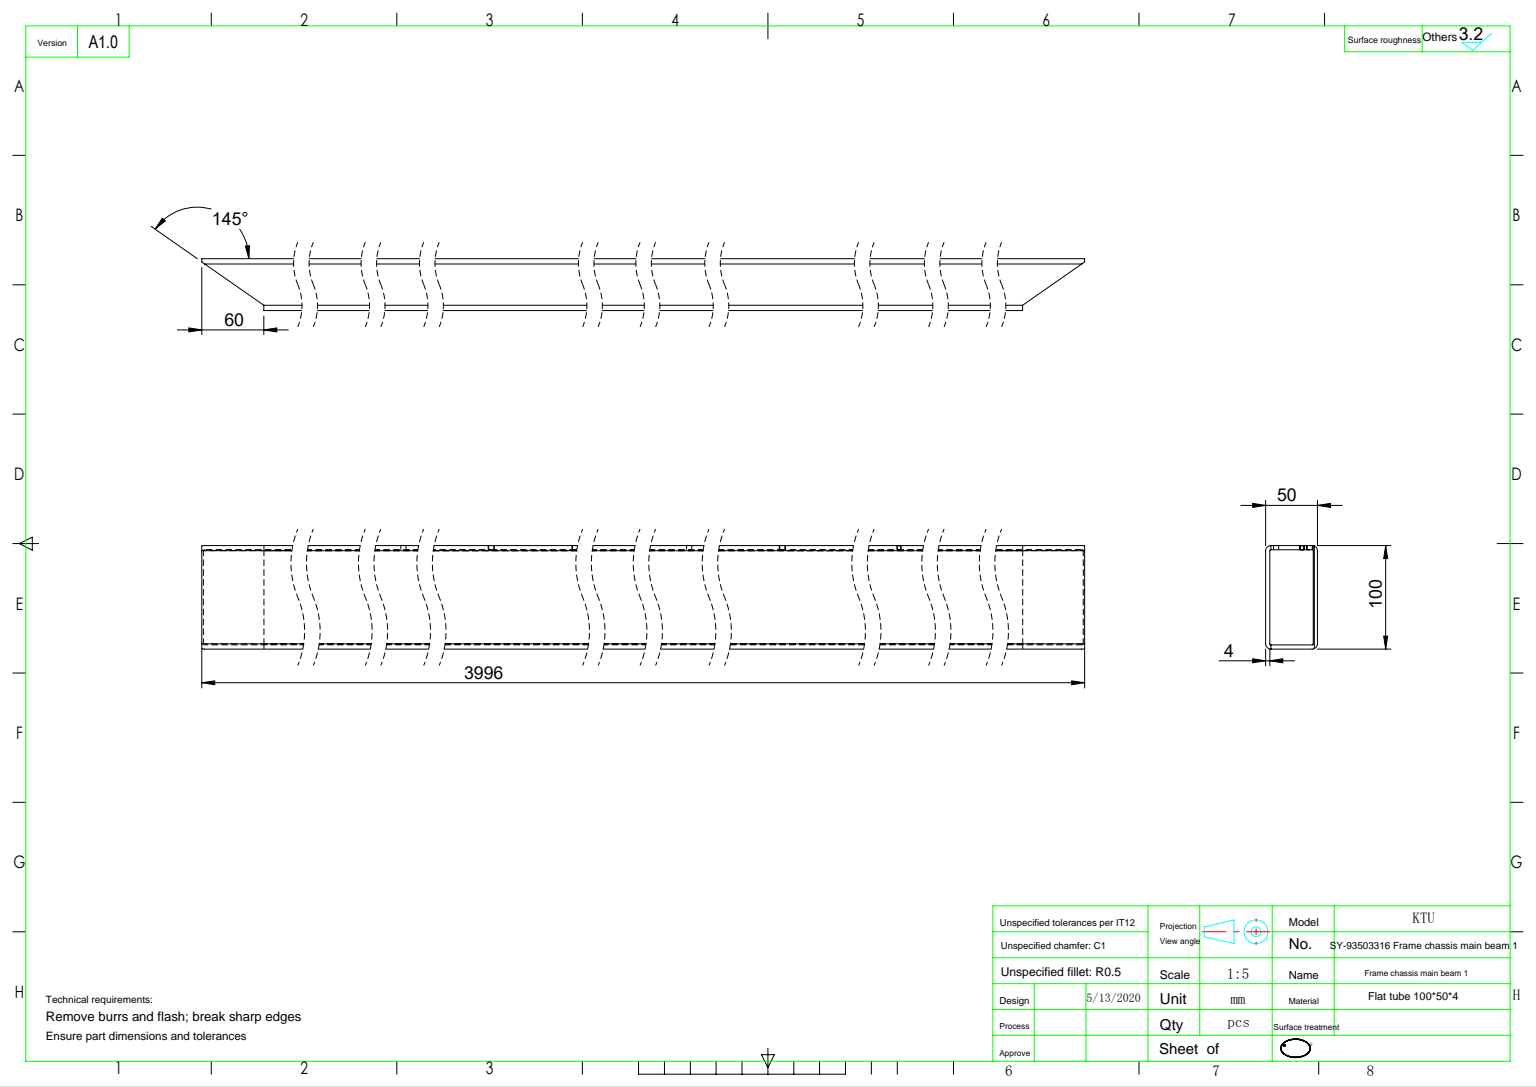
from build123d import *

# Parameters (mm, degrees)
EXTRUDE_1_DEPTH             = 1938
EXTRUDE_1_2_DEPTH           = 60
CUT_EXTRUDE_2_DEPTH         = 2001.657142041
EXTRUDE_2_DEPTH             = 60
CUT_EXTRUDE_3_DEPTH         = 2001.657142041
HOLE_WIZARD_M6_1_AT_2_COUNT = 2
HOLE_WIZARD_M6_1_AT_2_PITCH = 81
HOLE_WIZARD_M6_1_AT_3_COUNT = 2
HOLE_WIZARD_M6_1_AT_3_PITCH = 1168
HOLE_WIZARD_M6_1_AT_4_COUNT = 2
HOLE_WIZARD_M6_1_AT_4_PITCH = 1249
MM_1_AT_2_COUNT             = 2
MM_1_AT_2_PITCH             = 700
PATTERN_LINEAR_1_COUNT      = 3
PATTERN_LINEAR_1_PITCH      = 1168
HOLE_WIZARD_M4_1_AT_2_COUNT = 2
HOLE_WIZARD_M4_1_AT_2_PITCH = 530
HOLE_WIZARD_M4_1_AT_3_COUNT = 2
HOLE_WIZARD_M4_1_AT_3_PITCH = 550.506310809
HOLE_WIZARD_M4_1_AT_4_COUNT = 2
HOLE_WIZARD_M4_1_AT_4_PITCH = 871
HOLE_WIZARD_M4_1_AT_5_COUNT = 2
HOLE_WIZARD_M4_1_AT_5_PITCH = 1425
HOLE_WIZARD_M4_1_AT_6_COUNT = 2
HOLE_WIZARD_M4_1_AT_6_PITCH = 1446
HOLE_WIZARD_M4_1_AT_7_COUNT = 2
HOLE_WIZARD_M4_1_AT_7_PITCH = 1786
HOLE_WIZARD_M4_1_AT_8_COUNT = 2
HOLE_WIZARD_M4_1_AT_8_PITCH = 2321
SKETCH_20_R                 = 1.65
CUT_EXTRUDE_4_DEPTH         = 10


with BuildPart() as part:
    # 草图1 → Extrude 1 (new, symmetric)
    with BuildSketch(Plane.XY):
        with BuildLine():
            Line((-20, 50), (20, 50))
            ThreePointArc((20, 50), (23.535533906, 48.535533906), (25, 45))
            Line((25, 45), (25, -45))
            ThreePointArc((25, -45), (23.535533906, -48.535533906), (20, -50))
            Line((20, -50), (-20, -50))
            ThreePointArc((-20, -50), (-23.535533906, -48.535533906), (-25, -45))
            Line((-25, -45), (-25, 45))
            ThreePointArc((-25, 45), (-23.535533906, 48.535533906), (-20, 50))
        make_face()
        with BuildLine():
            Line((-20, 46), (20, 46))
            ThreePointArc((20, 46), (20.707106781, 45.707106781), (21, 45))
            Line((21, 45), (21, -45))
            ThreePointArc((21, -45), (20.707106781, -45.707106781), (20, -46))
            Line((20, -46), (-20, -46))
            ThreePointArc((-20, -46), (-20.707106781, -45.707106781), (-21, -45))
            Line((-21, -45), (-21, 45))
            ThreePointArc((-21, 45), (-20.707106781, 45.707106781), (-20, 46))
        make_face(mode=Mode.SUBTRACT)
    extrude(amount=EXTRUDE_1_DEPTH, both=True)

    # 草图12 → M6 螺纹孔1 (revolve, cut)
    with BuildSketch(Plane(origin=(-17.5, 50, -624.5), x_dir=(0, 0, 1), z_dir=(1, 0, 0))):
        Polygon((0, 0), (0, 16.502151548), (2.5, 15), (2.5, 0), align=None)
    hole_wizard_m6_1 = revolve(axis=Axis((-17.5, 56.35, -624.5), (0, -1, 0)), mode=Mode.SUBTRACT)

    # M6 螺纹孔1 at 2: M6 螺纹孔1 ×2
    with Locations(*[(0, 0, i * HOLE_WIZARD_M6_1_AT_2_PITCH) for i in range(1, HOLE_WIZARD_M6_1_AT_2_COUNT)]):
        add(hole_wizard_m6_1, mode=Mode.SUBTRACT)

    # M6 螺纹孔1 at 3: M6 螺纹孔1 ×2
    with Locations(*[(0, 0, i * HOLE_WIZARD_M6_1_AT_3_PITCH) for i in range(1, HOLE_WIZARD_M6_1_AT_3_COUNT)]):
        add(hole_wizard_m6_1, mode=Mode.SUBTRACT)

    # M6 螺纹孔1 at 4: M6 螺纹孔1 ×2
    with Locations(*[(0, 0, i * HOLE_WIZARD_M6_1_AT_4_PITCH) for i in range(1, HOLE_WIZARD_M6_1_AT_4_COUNT)]):
        add(hole_wizard_m6_1, mode=Mode.SUBTRACT)

    # 草图14 → 大小mm 暗销孔1 (revolve, cut)
    with BuildSketch(Plane(origin=(15, 50, -818), x_dir=(0, 0, 1), z_dir=(1, 0, 0))):
        Polygon((0, 0), (0, 10.002151548), (2.5, 8.5), (2.5, 0.025), (2.525, 0), align=None)
    mm_1 = revolve(axis=Axis((15, 56.35, -818), (0, -1, 0)), mode=Mode.SUBTRACT)

    # 大小mm 暗销孔1 at 2: 大小mm 暗销孔1 ×2
    with Locations(*[(0, 0, -i * MM_1_AT_2_PITCH) for i in range(1, MM_1_AT_2_COUNT)]):
        add(mm_1, mode=Mode.SUBTRACT)

    # 阵列(线性)1: 大小mm 暗销孔1 ×3
    with Locations(*[(0, 0, i * PATTERN_LINEAR_1_PITCH) for i in range(1, PATTERN_LINEAR_1_COUNT)]):
        add(mm_1, mode=Mode.SUBTRACT)

    # 阵列(线性)1 copy 1 sketch → 阵列(线性)1 copy 1 (revolve, cut)
    with BuildSketch(Plane(origin=(15, 50, -350), x_dir=(0, 0, 1), z_dir=(1, 0, 0))):
        Polygon((0, 0), (0, 10.002151548), (2.5, 8.5), (2.5, 0.025), (2.525, 0), align=None)
    revolve(axis=Axis((15, 56.35, -350), (0, -1, 0)), mode=Mode.SUBTRACT)

    # 阵列(线性)1 copy 2 sketch → 阵列(线性)1 copy 2 (revolve, cut)
    with BuildSketch(Plane(origin=(15, 50, 818), x_dir=(0, 0, 1), z_dir=(1, 0, 0))):
        Polygon((0, 0), (0, 10.002151548), (2.5, 8.5), (2.5, 0.025), (2.525, 0), align=None)
    revolve(axis=Axis((15, 56.35, 818), (0, -1, 0)), mode=Mode.SUBTRACT)

    # 草图17 → M4 螺纹孔1 (revolve, cut)
    with BuildSketch(Plane(origin=(-10, 50, 1628), x_dir=(0, 0, 1), z_dir=(1, 0, 0))):
        Polygon((0, 0), (0, 11.091420021), (1.65, 10.1), (1.65, 0.375), (2.025, 0), align=None)
    hole_wizard_m4_1 = revolve(axis=Axis((-10, 56.35, 1628), (0, -1, 0)), mode=Mode.SUBTRACT)

    # M4 螺纹孔1 at 2: M4 螺纹孔1 ×2
    with Locations(*[(0, 0, -i * HOLE_WIZARD_M4_1_AT_2_PITCH) for i in range(1, HOLE_WIZARD_M4_1_AT_2_COUNT)]):
        add(hole_wizard_m4_1, mode=Mode.SUBTRACT)

    # M4 螺纹孔1 at 3: M4 螺纹孔1 ×2
    with Locations(*[(0, 0, -i * HOLE_WIZARD_M4_1_AT_3_PITCH) for i in range(1, HOLE_WIZARD_M4_1_AT_3_COUNT)]):
        add(hole_wizard_m4_1, mode=Mode.SUBTRACT)

    # M4 螺纹孔1 at 4: M4 螺纹孔1 ×2
    with Locations(*[(0, 0, -i * HOLE_WIZARD_M4_1_AT_4_PITCH) for i in range(1, HOLE_WIZARD_M4_1_AT_4_COUNT)]):
        add(hole_wizard_m4_1, mode=Mode.SUBTRACT)

    # M4 螺纹孔1 at 5: M4 螺纹孔1 ×2
    with Locations(*[(0, 0, -i * HOLE_WIZARD_M4_1_AT_5_PITCH) for i in range(1, HOLE_WIZARD_M4_1_AT_5_COUNT)]):
        add(hole_wizard_m4_1, mode=Mode.SUBTRACT)

    # M4 螺纹孔1 at 6: M4 螺纹孔1 ×2
    with Locations(*[(0, 0, -i * HOLE_WIZARD_M4_1_AT_6_PITCH) for i in range(1, HOLE_WIZARD_M4_1_AT_6_COUNT)]):
        add(hole_wizard_m4_1, mode=Mode.SUBTRACT)

    # M4 螺纹孔1 at 7: M4 螺纹孔1 ×2
    with Locations(*[(0, 0, -i * HOLE_WIZARD_M4_1_AT_7_PITCH) for i in range(1, HOLE_WIZARD_M4_1_AT_7_COUNT)]):
        add(hole_wizard_m4_1, mode=Mode.SUBTRACT)

    # M4 螺纹孔1 at 8: M4 螺纹孔1 ×2
    with Locations(*[(0, 0, -i * HOLE_WIZARD_M4_1_AT_8_PITCH) for i in range(1, HOLE_WIZARD_M4_1_AT_8_COUNT)]):
        add(hole_wizard_m4_1, mode=Mode.SUBTRACT)

    # 草图19 → M4 螺纹孔2 (revolve, cut)
    with BuildSketch(Plane(origin=(-10, 50, -1453), x_dir=(0, 0, 1), z_dir=(1, 0, 0))):
        Polygon((0, 0), (0, 11.091420021), (1.65, 10.1), (1.65, 0.375), (2.025, 0), align=None)
    revolve(axis=Axis((-10, 56.35, -1453), (0, -1, 0)), mode=Mode.SUBTRACT)


with BuildPart() as body_2:
    # 草图7 → Extrude 1 2 (new body)
    with BuildSketch(Plane.XY.offset(1938)):
        with BuildLine():
            Line((25, -45), (25, 45))
            ThreePointArc((25, 45), (23.535533906, 48.535533906), (20, 50))
            Line((20, 50), (-20, 50))
            ThreePointArc((-20, 50), (-23.535533906, 48.535533906), (-25, 45))
            Line((-25, 45), (-25, -45))
            ThreePointArc((-25, -45), (-23.535533906, -48.535533906), (-20, -50))
            Line((-20, -50), (20, -50))
            ThreePointArc((20, -50), (23.535533906, -48.535533906), (25, -45))
        make_face()
        with BuildLine():
            Line((21, -45), (21, 45))
            ThreePointArc((21, 45), (20.707106781, 45.707106781), (20, 46))
            Line((20, 46), (-20, 46))
            ThreePointArc((-20, 46), (-20.707106781, 45.707106781), (-21, 45))
            Line((-21, 45), (-21, -45))
            ThreePointArc((-21, -45), (-20.707106781, -45.707106781), (-20, -46))
            Line((-20, -46), (20, -46))
            ThreePointArc((20, -46), (20.707106781, -45.707106781), (21, -45))
        make_face(mode=Mode.SUBTRACT)
    extrude(amount=EXTRUDE_1_2_DEPTH)

    # 草图8 → 切除-拉伸2 (cut, through all)
    with BuildSketch(Plane(origin=(0, 50, 0), x_dir=(1, 0, 0), z_dir=(0, 1, 0))):
        Polygon((20, -1938), (-22.012452293, -1998), (31.913764891, -1998), (31.913764891, -1938), align=None)
    extrude(amount=-CUT_EXTRUDE_2_DEPTH, mode=Mode.SUBTRACT)


with BuildPart() as body_3:
    # 草图9 → 凸台-拉伸2 (new body)
    with BuildSketch(Plane(origin=(0, 0, -1938), x_dir=(-1, 0, 0), z_dir=(0, 0, -1))):
        with BuildLine():
            Line((20, -50), (-20, -50))
            ThreePointArc((-20, -50), (-23.535533906, -48.535533906), (-25, -45))
            Line((-25, -45), (-25, 45))
            ThreePointArc((-25, 45), (-23.535533906, 48.535533906), (-20, 50))
            Line((-20, 50), (20, 50))
            ThreePointArc((20, 50), (23.535533906, 48.535533906), (25, 45))
            Line((25, 45), (25, -45))
            ThreePointArc((25, -45), (23.535533906, -48.535533906), (20, -50))
        make_face()
        with BuildLine():
            Line((-20, 46), (20, 46))
            ThreePointArc((20, 46), (20.707106781, 45.707106781), (21, 45))
            Line((21, 45), (21, -45))
            ThreePointArc((21, -45), (20.707106781, -45.707106781), (20, -46))
            Line((20, -46), (-20, -46))
            ThreePointArc((-20, -46), (-20.707106781, -45.707106781), (-21, -45))
            Line((-21, -45), (-21, 45))
            ThreePointArc((-21, 45), (-20.707106781, 45.707106781), (-20, 46))
        make_face(mode=Mode.SUBTRACT)
    extrude(amount=EXTRUDE_2_DEPTH)

    # 草图10 → 切除-拉伸3 (cut, through all)
    with BuildSketch(Plane(origin=(0, 50, 0), x_dir=(1, 0, 0), z_dir=(0, 1, 0))):
        Polygon((20, 1938), (-22.012452293, 1998), (25, 1998), (25, 1938), align=None)
    extrude(amount=-CUT_EXTRUDE_3_DEPTH, mode=Mode.SUBTRACT)

    # Combine 1: union part
    add(part.part)

    # Combine 2: union body 2
    add(body_2.part)

    # 草图20 → 切除-拉伸4 (cut)
    with BuildSketch(Plane(origin=(0, 50, 0), x_dir=(1, 0, 0), z_dir=(0, 1, 0))):
        with Locations(Location((-10, 1710, 0), (0, 0, 270))):
            Circle(SKETCH_20_R)
    extrude(amount=-CUT_EXTRUDE_4_DEPTH, mode=Mode.SUBTRACT)


solid = body_3.part
